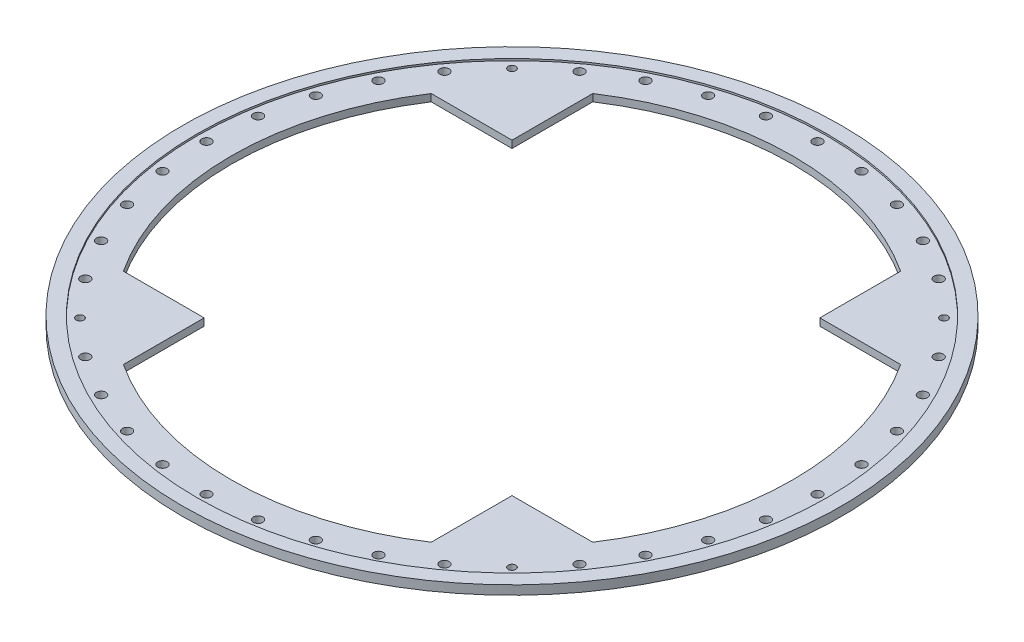
from build123d import *

# Parameters (mm, degrees)
SKETCH_1_R               = 910
EXTRUDE_1_DEPTH          = 25
SKETCH_2_R               = 870
CUT_EXTRUDE_1_DEPTH      = 5
HOLE_WIZARD_26_1_D       = 26
PATTERN_CIRCULAR_1_COUNT = 40
HOLE_WIZARD_M24_1_D      = 21


with BuildPart() as part:
    # 草图1 → 凸台-拉伸1 (new body)
    with BuildSketch(Plane(origin=(0, 0, 0), x_dir=(1, 0, 0), z_dir=(0, 1, 0))):
        with Locations(Location((0, 0, 0), (0, 0, 270))):
            Circle(SKETCH_1_R)
        with BuildLine():
            Line((-648.074069841, 425), (-425, 425))
            Line((-425, 425), (-425, 648.074069841))
            ThreePointArc((-425, 648.074069841), (0, 775), (425, 648.074069841))
            Line((425, 648.074069841), (425, 425))
            Line((425, 425), (648.074069841, 425))
            ThreePointArc((648.074069841, 425), (775, 0), (648.074069841, -425))
            Line((648.074069841, -425), (425, -425))
            Line((425, -425), (425, -648.074069841))
            ThreePointArc((425, -648.074069841), (0, -775), (-425, -648.074069841))
            Line((-425, -648.074069841), (-425, -425))
            Line((-425, -425), (-648.074069841, -425))
            ThreePointArc((-648.074069841, -425), (-775, 0), (-648.074069841, 425))
        make_face(mode=Mode.SUBTRACT)
    extrude(amount=EXTRUDE_1_DEPTH)

    # 草图2 → 切除-拉伸1 (cut)
    with BuildSketch(Plane(origin=(0, 25, 0), x_dir=(1, 0, 0), z_dir=(0, 1, 0))):
        with Locations(Location((0, 0, 0), (0, 0, 270))):
            Circle(SKETCH_2_R)
    extrude(amount=-CUT_EXTRUDE_1_DEPTH, mode=Mode.SUBTRACT)

    # Ø26 直径孔1 (through all)
    with Locations(Plane(origin=(0, 20, 0), x_dir=(1, 0, 0), z_dir=(0, 1, 0))):
        with Locations((0, 843.5)):
            hole_wizard_26_1 = Hole(HOLE_WIZARD_26_1_D / 2)

    # 阵列(圆周)1: Ø26 直径孔1 ×40 about axis, 4 skipped
    pattern_circular_1_axis = Axis((0, 0, 0), (0, 1, 0))
    add([hole_wizard_26_1.rotate(pattern_circular_1_axis, i * 360 / PATTERN_CIRCULAR_1_COUNT) for i in range(1, PATTERN_CIRCULAR_1_COUNT) if i not in (5, 15, 25, 35)], mode=Mode.SUBTRACT)

    # M24 螺纹孔1 (through all)
    with Locations(Plane(origin=(0, 20, 0), x_dir=(1, 0, 0), z_dir=(0, 1, 0))):
        with Locations((-596.444569931, 596.444569931), (596.444569931, 596.444569931), (596.444569931, -596.444569931), (-596.444569931, -596.444569931)):
            Hole(HOLE_WIZARD_M24_1_D / 2)


solid = part.part
